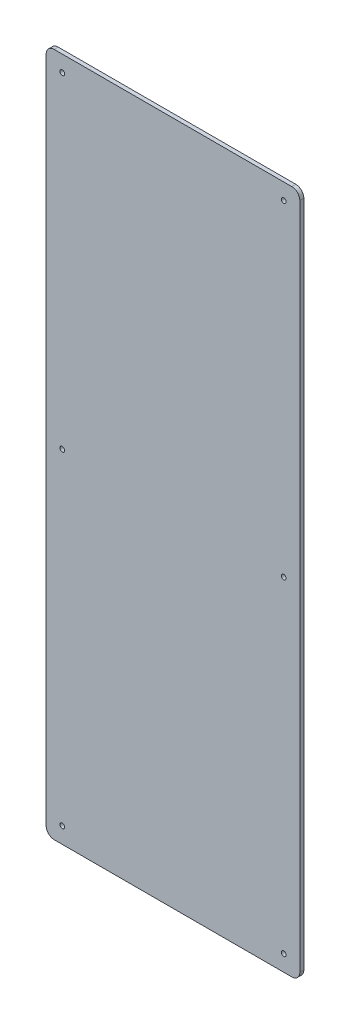
SolidWorks part; units mm, degrees
material "PMMA（透明）"
ref_plane "前视基准面" through (0, 0, 0) normal (0, 0, 1) x (1, 0, 0)
ref_plane "上视基准面" through (0, 0, 0) normal (0, 1, 0) x (1, 0, 0)
ref_plane "右视基准面" through (0, 0, 0) normal (1, 0, 0) x (0, 0, -1)
sketch "草图1" plane through (0, 0, 0) normal (0, 0, 1) x (1, 0, 0)
  line L1 (-157.5, -425) -> (157.5, -425)
  line L2 (-157.5, -425) -> (-157.5, 425)
  line L3 (-157.5, 425) -> (157.5, 425)
  line L4 (157.5, -425) -> (157.5, 425)
  line L5 (-157.5, -425) -> (157.5, 425) construction
  line L6 (-157.5, 425) -> (157.5, -425) construction
  point P0 (0, 0)
  dimension "D1" = 315
  dimension "D2" = 850
extrude "凸台-拉伸1" add sketch "草图1" along normal blind 5
hole_wizard "Ø6.0 (6) 直径孔1" positions "草图2" profile "草图3" hole size "Ø6.0" standard "ISO"
sketch "草图2" plane through (0, 0, 5) normal (0, 0, 1) x (1, 0, 0)
  line L0 (-157.5, 0) -> (157.5, 0) construction
  line L1 (-157.5, 425) -> (-157.5, -425) construction
  line L2 (157.5, -425) -> (157.5, 425) construction
  line L4 (0, 425) -> (0, -425) construction
  line L5 (157.5, 425) -> (-157.5, 425) construction
  line L6 (-157.5, -425) -> (157.5, -425) construction
  point P0 (-137.5, 405)
  point P2 (137.5, 405)
  point P21 (137.5, -405)
  point P22 (-137.5, -405)
  point P23 (-137.5, 0)
  point P27 (137.5, 0)
  dimension "D1" = 20
  dimension "D2" = 20
sketch "草图3" plane through (-137.5, 405, 5) normal (1, 0, 0) x (0, -1, 0)
  line L0 (0, 0) -> (0, 29.5526)
  line L1 (0, 29.5526) -> (3, 27.75)
  line L2 (3, 27.75) -> (3, 0)
  line L5 (3, 0) -> (0, 0)
  line L10 (0, 29.5526) -> (-3, 27.75) construction
  line L11 (0, -6.35) -> (0, 107.95) construction
  dimension "孔直径" = 6
  dimension "孔深度" = 27.75
  dimension "导头角度" = 118
fillet "圆角1" radius 10 4 edges at (-157.5, -425, 2.5) (157.5, -425, 2.5) (157.5, 425, 2.5) (-157.5, 425, 2.5)
